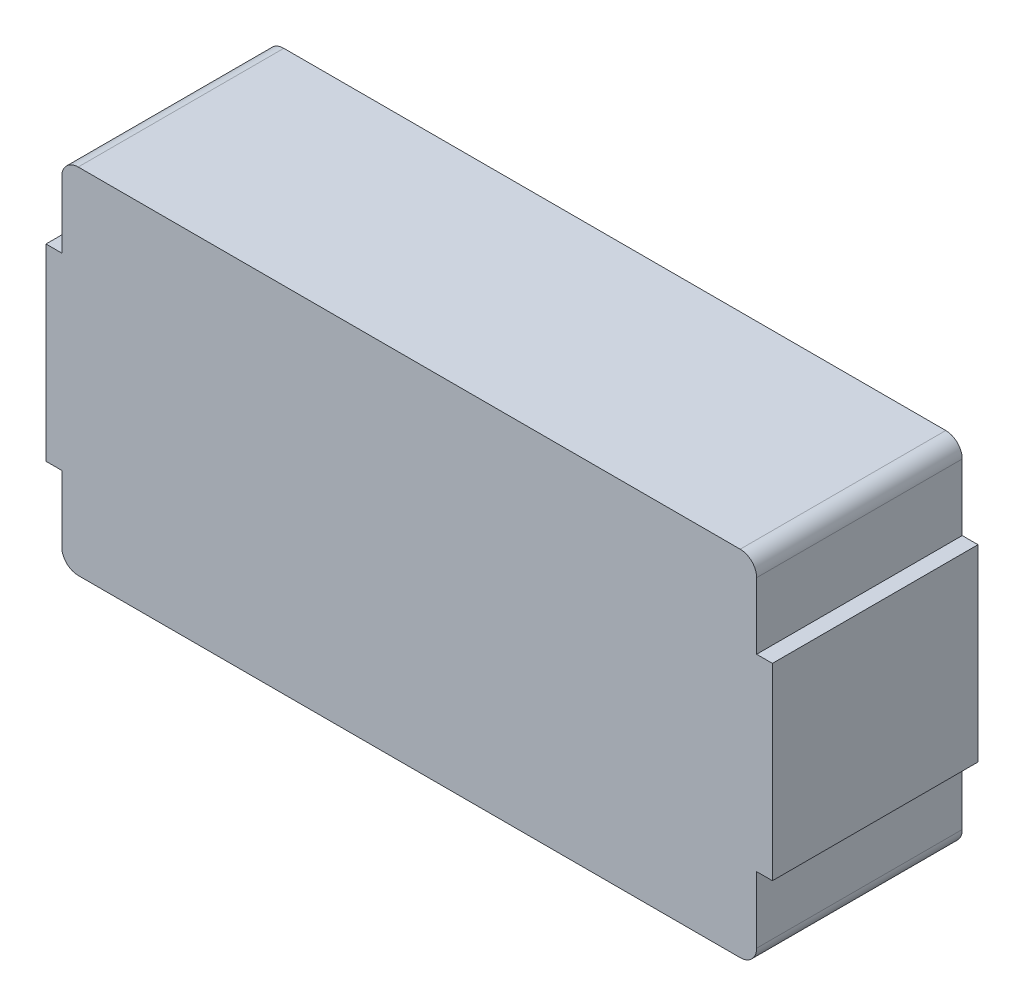
SolidWorks part; units mm, degrees
ref_plane "Front Plane" through (0, 0, 0) normal (0, 0, 1) x (1, 0, 0)
ref_plane "Top Plane" through (0, 0, 0) normal (0, 1, 0) x (1, 0, 0)
ref_plane "Right Plane" through (0, 0, 0) normal (1, 0, 0) x (0, 0, -1)
other "Configuration Table"
sketch "Sketch1" plane through (0, 0, 0) normal (0, 0, 1) x (1, 0, 0)
  line L0 (27.0657, 0) -> (-27.1889, 0) construction
  line L1 (27.0657, -12.4829) -> (-27.1889, -12.4829)
  line L2 (27.0657, 12.4829) -> (-27.1889, 12.4829)
  arc A0 (27.0657, -12.4829) -> (27.0657, 12.4829) centre (27.0657, 0) ccw
  arc A1 (-27.1889, 12.4829) -> (-27.1889, -12.4829) centre (-27.1889, 0) ccw
  point P2 (-0.0616, 0)
extrude "Boss-Extrude1" add sketch "Sketch1" along normal blind 4
sketch "Sketch2" plane through (0, 0, 4) normal (0, 0, 1) x (1, 0, 0)
  line L0 (0, -21.5109) -> (0, -37.0864) construction
  line L1 (42.2492, -21.5109) -> (-42.2492, -21.5109)
  line L2 (42.2492, -21.5109) -> (42.2492, -11.4452)
  line L3 (42.2492, 21.5109) -> (-42.2492, 21.5109)
  line L4 (-42.2492, -21.5109) -> (-42.2492, -11.4452)
  line L5 (42.2492, -21.5109) -> (-42.2492, 21.5109) construction
  line L6 (42.2492, 21.5109) -> (-42.2492, -21.5109) construction
  line L7 (44.1675, -11.4452) -> (42.2492, -11.4452)
  line L8 (44.1675, -11.4452) -> (44.1675, 11.4452)
  line L9 (44.1675, 11.4452) -> (42.2492, 11.4452)
  line L11 (-44.1675, 11.4452) -> (-42.2492, 11.4452)
  line L12 (-44.1675, -11.4452) -> (-44.1675, 11.4452)
  line L13 (-44.1675, -11.4452) -> (-42.2492, -11.4452)
  line L14 (42.2492, 11.4452) -> (42.2492, 21.5109)
  line L15 (-42.2492, 11.4452) -> (-42.2492, 21.5109)
  point P0 (42.2492, 0)
  point P15 (-42.2492, 0)
extrude "Boss-Extrude2" add sketch "Sketch2" along normal blind 25
fillet "Fillet1" radius 2 4 edges at (-42.2492, 21.5109, 16.5) (-42.2492, -21.5109, 16.5) (42.2492, 21.5109, 16.5) (42.2492, -21.5109, 16.5)
